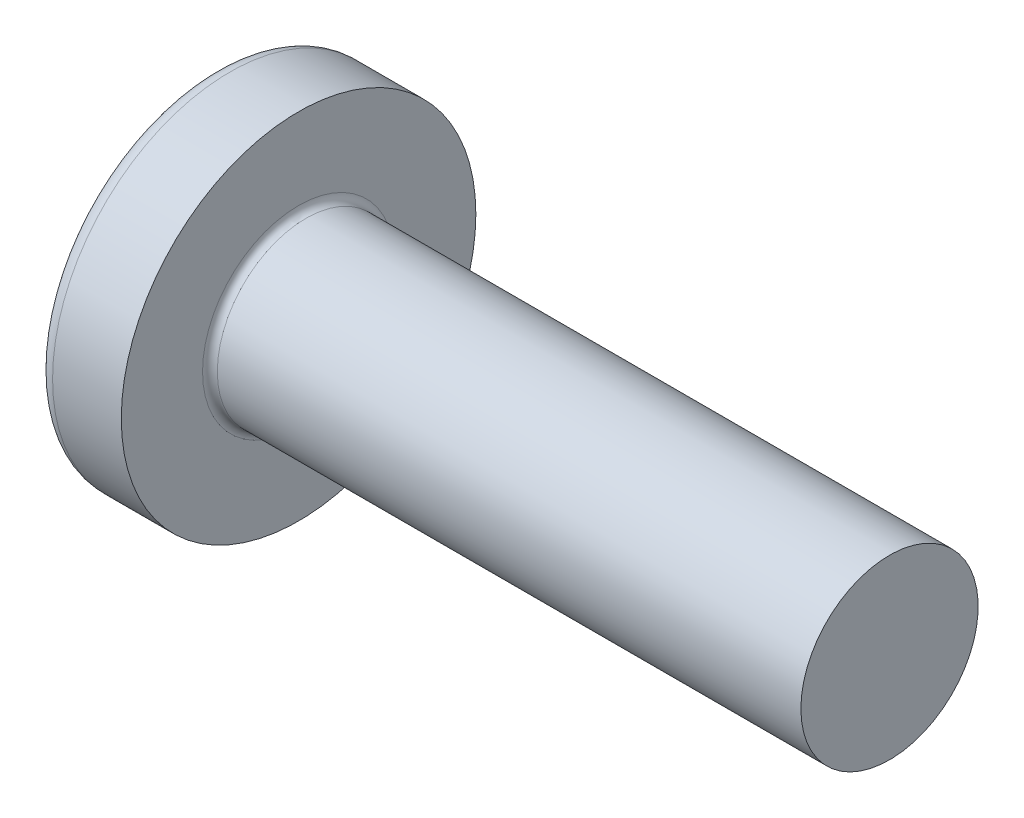
from build123d import *

# Parameters (mm, degrees)
FILLET1_R    = 0.25
RECPAT_COUNT = 2
RECPAT_ANGLE = 90


with BuildPart() as part:
    # BodySke → BaseBody (revolve)
    with BuildSketch(Plane.XY, mode=Mode.PRIVATE) as basebody_sk:
        with BuildLine():
            Line((0, 0), (24.6, 0))
            Line((24.6, 0), (24.6, 3))
            Line((24.6, 3), (4.6, 3))
            Line((4.6, 3), (4.6, 6))
            Line((4.6, 6), (2.274716834, 6))
            ThreePointArc((2.274716834, 6), (2.026424569, 5.939532013), (1.833738725, 5.77167019))
            ThreePointArc((1.833738725, 5.77167019), (0.469454036, 3.027985077), (0, 0))
        make_face()
    revolve(basebody_sk.sketch.rotate(Axis((0, 0, 0), (1, 0, 0)), 90), axis=Axis((0, 0, 0), (1, 0, 0)))

    # Fillet1
    fillet1_edges = [part.edges().sort_by_distance(p)[0] for p in [
        (4.6, 0, -3),
    ]]
    fillet(fillet1_edges, radius=FILLET1_R)

    # RecessTopSke → Recess section 0
    with BuildSketch(Plane(origin=(0, 0, 0), x_dir=(0, 0, -1), z_dir=(1, 0, 0))):
        with BuildLine():
            Line((-0.71, 3.35), (0.71, 3.35))
            Line((0.71, 3.35), (0.71, -3.35))
            Line((0.71, -3.35), (-0.71, -3.35))
            Line((-0.71, -3.35), (-0.71, 3.35))
        make_face()
    # RecessBottomSke → Recess section 1
    with BuildSketch(Plane(origin=(3.46, 0, 0), x_dir=(0, 0, -1), z_dir=(1, 0, 0))):
        with BuildLine():
            Line((-0.71, -1.4405), (0.71, -1.4405))
            Line((0.71, -1.4405), (0.71, 1.4405))
            Line((0.71, 1.4405), (-0.71, 1.4405))
            Line((-0.71, 1.4405), (-0.71, -1.4405))
        make_face()
    recess = loft(mode=Mode.SUBTRACT)

    # RecPat: Recess ×2 about axis
    recpat_axis = Axis((0, 0, 0), (1, 0, 0))
    for i in range(1, RECPAT_COUNT):
        add(recess.rotate(recpat_axis, i * RECPAT_ANGLE / (RECPAT_COUNT - 1)), mode=Mode.SUBTRACT)

    # RecessCoreSke → RecessCore (revolve, cut)
    with BuildSketch(Plane.XY, mode=Mode.PRIVATE) as recesscore_sk:
        Polygon((0, 0), (3.876059671, 0), (3.46, 1.2805), (0, 1.522446769), align=None)
    revolve(recesscore_sk.sketch.rotate(Axis((0, 0, 0), (1, 0, 0)), 346.974156952), axis=Axis((0, 0, 0), (1, 0, 0)), mode=Mode.SUBTRACT)


solid = part.part
